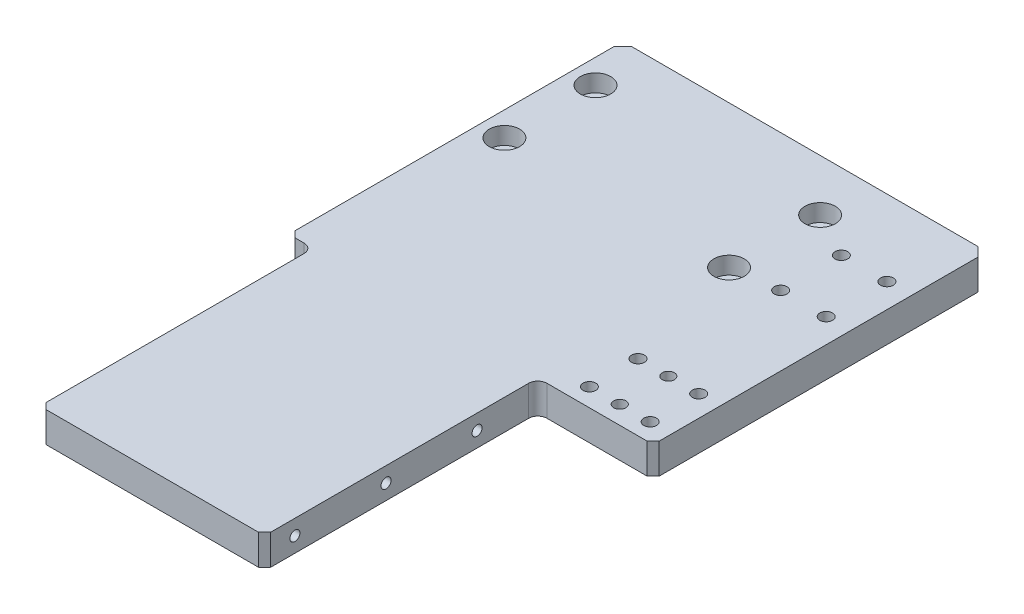
from build123d import *

# Parameters (mm, degrees)
SKETCH_1_W                = 120
SKETCH_1_H                = 200
EXTRUDE_1_DEPTH           = 10
CHAMFER_1_SIZE            = 3
HOLE_WIZARD_0_D           = 5.5
HOLE_WIZARD_0_DEPTH       = 10.1
HOLE_WIZARD_0_CBORE_D     = 10
HOLE_WIZARD_0_CBORE_DEPTH = 5.7
HOLE_WIZARD_0_TIP         = 1.652366702
SKETCH_4_W                = 38
SKETCH_4_H                = 90
SKETCH_4_W_2              = 8
CUT_EXTRUDE_1_DEPTH       = 20
CHAMFER_2_SIZE            = 2
FILLET_1_R                = 3
HOLE_WIZARD_M4_1_D        = 3.3
HOLE_WIZARD_M4_1_DEPTH    = 10.1
HOLE_WIZARD_M4_1_TIP      = 0.991420021
HOLE_WIZARD_M4_2_D        = 3.3
HOLE_WIZARD_M4_2_DEPTH    = 10.1
HOLE_WIZARD_M4_2_TIP      = 0.991420021
MM_2_D                    = 4
MM_2_DEPTH                = 12.4
MM_2_TIP                  = 1.201721238
HOLE_WIZARD_M5_2_D        = 4.2
HOLE_WIZARD_M5_2_DEPTH    = 12.4
HOLE_WIZARD_M5_2_TIP      = 1.2618073
HOLE_WIZARD_M5_3_D        = 4.2
HOLE_WIZARD_M5_3_DEPTH    = 12.4
HOLE_WIZARD_M5_3_TIP      = 1.2618073


with BuildPart() as part:
    # 草图1 → 凸台-拉伸1 (new body)
    with BuildSketch(Plane(origin=(0, 0, 0), x_dir=(1, 0, 0), z_dir=(0, 1, 0))):
        Rectangle(SKETCH_1_W, SKETCH_1_H)
    extrude(amount=EXTRUDE_1_DEPTH)

    # 倒角1
    chamfer_1_edges = [part.edges().sort_by_distance(p)[0] for p in [
        (60, 5, 100),
        (-60, 5, 100),
        (-60, 5, -100),
        (60, 5, -100),
    ]]
    chamfer(chamfer_1_edges, length=CHAMFER_1_SIZE)

    # 打孔尺寸(%根据)内六角圆柱头螺钉的类型0
    with Locations(Plane(origin=(0, 10, 0), x_dir=(1, 0, 0), z_dir=(0, 1, 0))):
        with Locations((-52, 83), (-52, 53), (22, 53), (22, 83)):
            CounterBoreHole(HOLE_WIZARD_0_D / 2, HOLE_WIZARD_0_CBORE_D / 2, HOLE_WIZARD_0_CBORE_DEPTH, depth=HOLE_WIZARD_0_DEPTH)
            with Locations((0, 0, -(HOLE_WIZARD_0_DEPTH + HOLE_WIZARD_0_TIP / 2))):  # 118° drill point
                Cone(0, HOLE_WIZARD_0_D / 2, HOLE_WIZARD_0_TIP, mode=Mode.SUBTRACT)

    # 草图4 → 切除-拉伸1 (cut)
    with BuildSketch(Plane(origin=(0, 10, 0), x_dir=(1, 0, 0), z_dir=(0, 1, 0))):
        with Locations((41, -55)):
            Rectangle(SKETCH_4_W, SKETCH_4_H)
        with Locations((-56, -55)):
            Rectangle(SKETCH_4_W_2, SKETCH_4_H)
    extrude(amount=-CUT_EXTRUDE_1_DEPTH, mode=Mode.SUBTRACT)

    # 倒角2
    chamfer_2_edges = [part.edges().sort_by_distance(p)[0] for p in [
        (22, 5, 100),
        (60, 5, 10),
        (-60, 5, 10),
        (-52, 5, 100),
    ]]
    chamfer(chamfer_2_edges, length=CHAMFER_2_SIZE)

    # 圆角1
    fillet_1_edges = [part.edges().sort_by_distance(p)[0] for p in [
        (22, 5, 10),
        (-52, 5, 10),
    ]]
    fillet(fillet_1_edges, radius=FILLET_1_R)

    # M4 螺纹孔1
    with Locations(Plane.ZY.offset(52)):
        with Locations((30, 5), (60, 5), (90, 5)):
            Hole(HOLE_WIZARD_M4_1_D / 2, depth=HOLE_WIZARD_M4_1_DEPTH)
            with Locations((0, 0, -(HOLE_WIZARD_M4_1_DEPTH + HOLE_WIZARD_M4_1_TIP / 2))):  # 118° drill point
                Cone(0, HOLE_WIZARD_M4_1_D / 2, HOLE_WIZARD_M4_1_TIP, mode=Mode.SUBTRACT)

    # M4 螺纹孔2
    with Locations(Plane(origin=(22, 0, 0), x_dir=(0, 0, -1), z_dir=(1, 0, 0))):
        with Locations((-30, 5), (-60, 5), (-90, 5)):
            Hole(HOLE_WIZARD_M4_2_D / 2, depth=HOLE_WIZARD_M4_2_DEPTH)
            with Locations((0, 0, -(HOLE_WIZARD_M4_2_DEPTH + HOLE_WIZARD_M4_2_TIP / 2))):  # 118° drill point
                Cone(0, HOLE_WIZARD_M4_2_D / 2, HOLE_WIZARD_M4_2_TIP, mode=Mode.SUBTRACT)

    # 大小mm 暗销孔2
    with Locations(Plane(origin=(0, 10, 0), x_dir=(1, 0, 0), z_dir=(0, 1, 0))):
        with Locations((43, 12), (43, -4)):
            Hole(MM_2_D / 2, depth=MM_2_DEPTH)
            with Locations((0, 0, -(MM_2_DEPTH + MM_2_TIP / 2))):  # 118° drill point
                Cone(0, MM_2_D / 2, MM_2_TIP, mode=Mode.SUBTRACT)

    # M5 螺纹孔2
    with Locations(Plane(origin=(0, 10, 0), x_dir=(1, 0, 0), z_dir=(0, 1, 0))):
        with Locations((53, -4), (33, -4), (53, 12), (33, 12)):
            Hole(HOLE_WIZARD_M5_2_D / 2, depth=HOLE_WIZARD_M5_2_DEPTH)
            with Locations((0, 0, -(HOLE_WIZARD_M5_2_DEPTH + HOLE_WIZARD_M5_2_TIP / 2))):  # 118° drill point
                Cone(0, HOLE_WIZARD_M5_2_D / 2, HOLE_WIZARD_M5_2_TIP, mode=Mode.SUBTRACT)

    # M5 螺纹孔3
    with Locations(Plane(origin=(0, 10, 0), x_dir=(1, 0, 0), z_dir=(0, 1, 0))):
        with Locations((52, 55), (37, 55), (52, 75), (37, 75)):
            Hole(HOLE_WIZARD_M5_3_D / 2, depth=HOLE_WIZARD_M5_3_DEPTH)
            with Locations((0, 0, -(HOLE_WIZARD_M5_3_DEPTH + HOLE_WIZARD_M5_3_TIP / 2))):  # 118° drill point
                Cone(0, HOLE_WIZARD_M5_3_D / 2, HOLE_WIZARD_M5_3_TIP, mode=Mode.SUBTRACT)


solid = part.part
